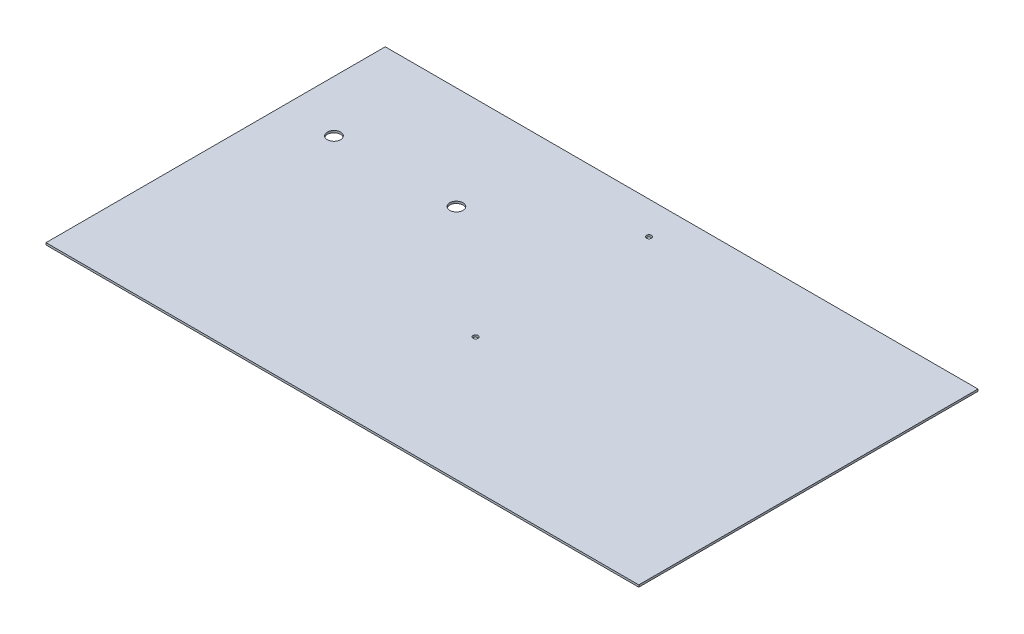
SolidWorks part; units mm, degrees
material "A3"
ref_plane "前视基准面" through (0, 0, 0) normal (0, 0, 1) x (1, 0, 0)
ref_plane "上视基准面" through (0, 0, 0) normal (0, 1, 0) x (1, 0, 0)
ref_plane "右视基准面" through (0, 0, 0) normal (1, 0, 0) x (0, 0, -1)
sketch "草图1" plane through (0, 0, 0) normal (0, 1, 0) x (1, 0, 0)
  line L0 (-235, 665) -> (-235, -665) construction
  line L1 (-1162, -665) -> (1162, -665)
  line L2 (-1162, -665) -> (-1162, 665)
  line L3 (-1162, 665) -> (1162, 665)
  line L4 (1162, -665) -> (1162, 665)
  line L5 (-1162, -665) -> (1162, 665) construction
  line L6 (-1162, 665) -> (1162, -665) construction
  line L7 (0, 665) -> (0, 0) construction
  line L9 (-1162, 505) -> (1162, 505) construction
  line L10 (-1162, 335) -> (1162, 335) construction
  line L11 (-1162, 147) -> (1162, 147) construction
  circle A2 centre (-480, 262) radius 26
  circle A3 centre (0, 537) radius 10
  circle A4 centre (0, -143) radius 10
  circle A5 centre (-960, 262) radius 26
  point P0 (0, 0)
  dimension "D6" = 20
  dimension "D8" = 235
  dimension "D9" = 52
  dimension "D11" = 480
  dimension "D7" = 128
  dimension "D12" = 680
  dimension "D13" = 52
  dimension "D14" = 480
  dimension "D1" = 1330
  dimension "D2" = 2324
  dimension "D3" = 160
  dimension "D4" = 330
  dimension "D5" = 188
  dimension "D10" = 403
extrude "凸台-拉伸1" add sketch "草图1" along normal mid plane 8
